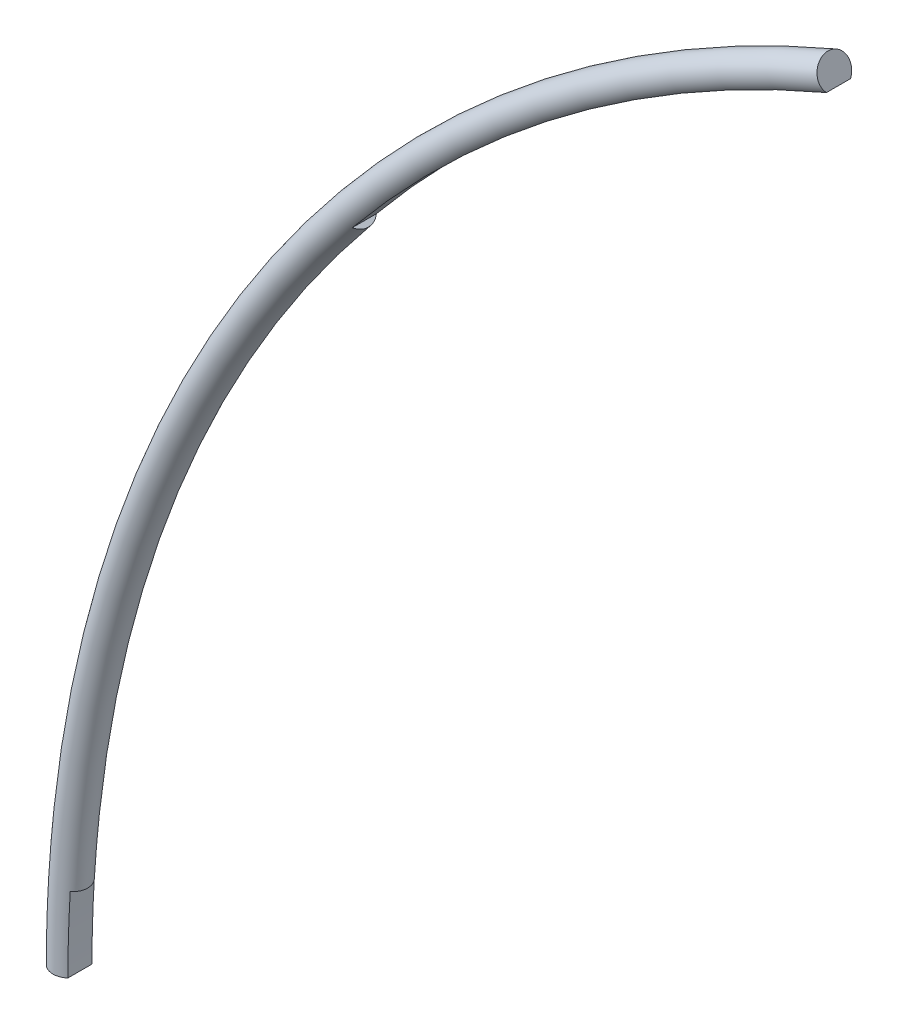
from build123d import *

# Parameters (mm, degrees)
SWEEP1_PROFILE_R   = 3
CUT_EXTRUDE1_DEPTH = 25


with BuildPart() as part:
    # Sweep1: sweep along a path in Sketch1
    with BuildLine(Plane.XY) as sweep1_path:
        ThreePointArc((-91.040352938, 214.477630854), (-194.295396542, 128.601317578), (-233, 0))
    # Sweep1 profile (on start of the path) → Sweep1 (sweep)
    with BuildSketch(Plane(origin=(-91.040352938, 214.477630854, 0), x_dir=(0.39073112848927155, -0.9205048534524413, 0), z_dir=(-0.9205048534524413, -0.39073112848927155, 0))):
        Circle(SWEEP1_PROFILE_R)
    sweep(path=sweep1_path.line)

    # Sketch6 → Cut-Extrude1 (cut, symmetric)
    with BuildSketch(Plane.XY):
        with BuildLine():
            Line((0, 0), (-230.569138435, 14.102212633))
            ThreePointArc((-230.569138435, 14.102212633), (-230.892259483, 7.054396551), (-231, 0))
            Line((-231, 0), (0, 0))
        make_face()
        with BuildLine():
            Line((0, 0), (-90.258890681, 212.636621148))
            ThreePointArc((-90.258890681, 212.636621148), (-138.212982732, 185.089630732), (-178.245278763, 146.934068884))
            Line((-178.245278763, 146.934068884), (0, 0))
        make_face()
    extrude(amount=CUT_EXTRUDE1_DEPTH, both=True, mode=Mode.SUBTRACT)


solid = part.part
